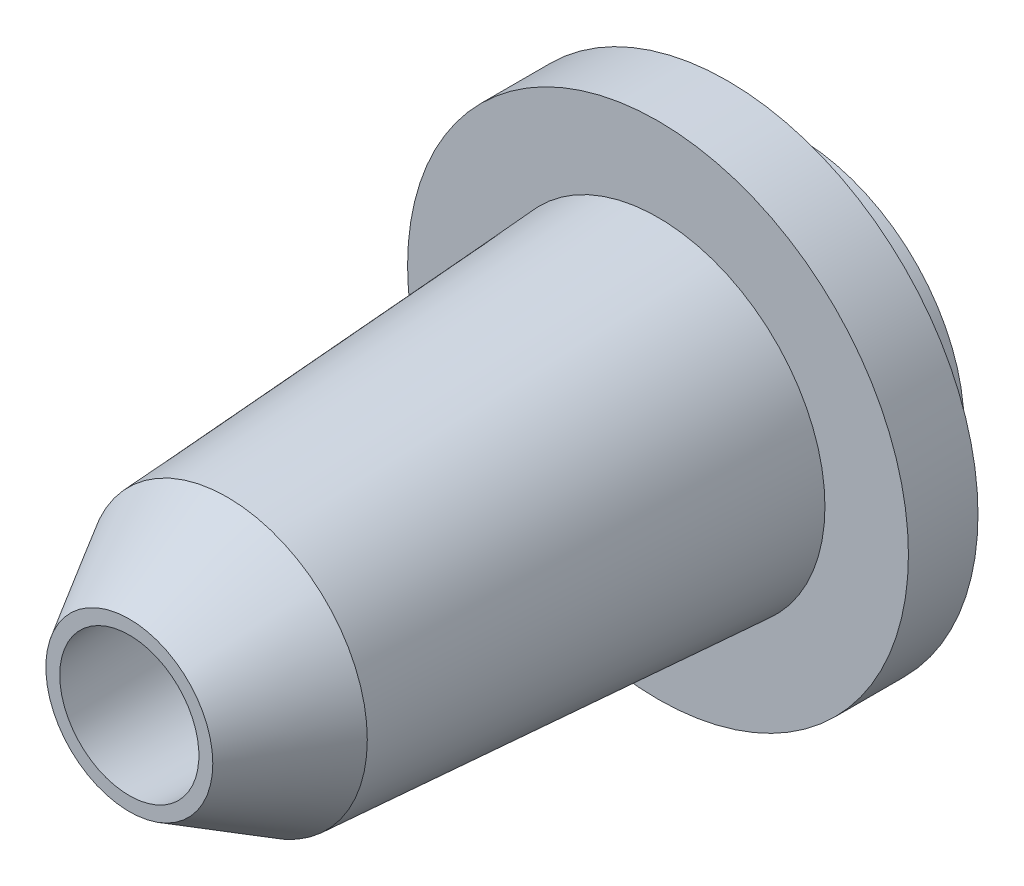
SolidWorks part; units mm, degrees
ref_plane "Front Plane" through (0, 0, 0) normal (0, 0, 1) x (1, 0, 0)
ref_plane "Top Plane" through (0, 0, 0) normal (0, 1, 0) x (1, 0, 0)
ref_plane "Right Plane" through (0, 0, 0) normal (1, 0, 0) x (0, 0, -1)
other "Configuration Table"
sketch "Sketch1" plane through (0, 0, 0) normal (0, 0, 1) x (1, 0, 0)
  circle A0 centre (0, 0) radius 12
  dimension "D1" = 24
extrude "Boss-Extrude1" add sketch "Sketch1" along normal blind 5
sketch "Sketch2" plane through (0, 0, 5) normal (0, 0, 1) x (1, 0, 0)
  circle A0 centre (0, 0) radius 18
  dimension "D1" = 36
extrude "Boss-Extrude2" add sketch "Sketch2" along normal blind 5
sketch "Sketch3" plane through (0, 0, 0) normal (1, 0, 0) x (0, 0, -1)
  line L0 (-10, 0) -> (-10, 12)
  line L1 (-10, 18) -> (-10, -18) construction
  line L2 (-10, 12) -> (-40.9591, 10.0651)
  line L3 (-40.9591, 10.0651) -> (-48, 6)
  line L4 (-48, 6) -> (-48, 0)
  line L5 (-48, 0) -> (-10, 0)
  line L6 (-40.9591, 10.0651) -> (-32.9591, 10.0651) construction
  line L7 (-32.9591, 10.0651) -> (-32.9591, 10.5651) construction
  dimension "D1" = 30
  dimension "D2" = 6
  dimension "D3" = 38
  dimension "D4" = 12
  dimension "D5" = 8
  dimension "D6" = 0.5
revolve "Revolve1" add sketch "Sketch3" angle 360 about L5
sketch "Sketch5" plane through (0, 0, 0) normal (0, 1, 0) x (1, 0, 0)
  line L0 (0, 0) -> (0, -48) construction
  line L1 (-6, -48) -> (6, -48) construction
  line L2 (0, -48) -> (5, -48)
  line L3 (5, -48) -> (8, 0)
  line L4 (12, 0) -> (-12, 0) construction
  line L5 (8, 0) -> (0, 0)
  line L6 (5, -48) -> (5, -40) construction
  line L7 (5, -40) -> (5.5, -40) construction
  line L8 (10.0651, -40.9591) -> (12, -10) construction
  line L9 (0, 0) -> (0, -48)
  dimension "D1" = 0.5
  dimension "D2" = 8
  dimension "D3" = 5
revolve "Cut-Revolve1" cut sketch "Sketch5" angle 360 about L9
